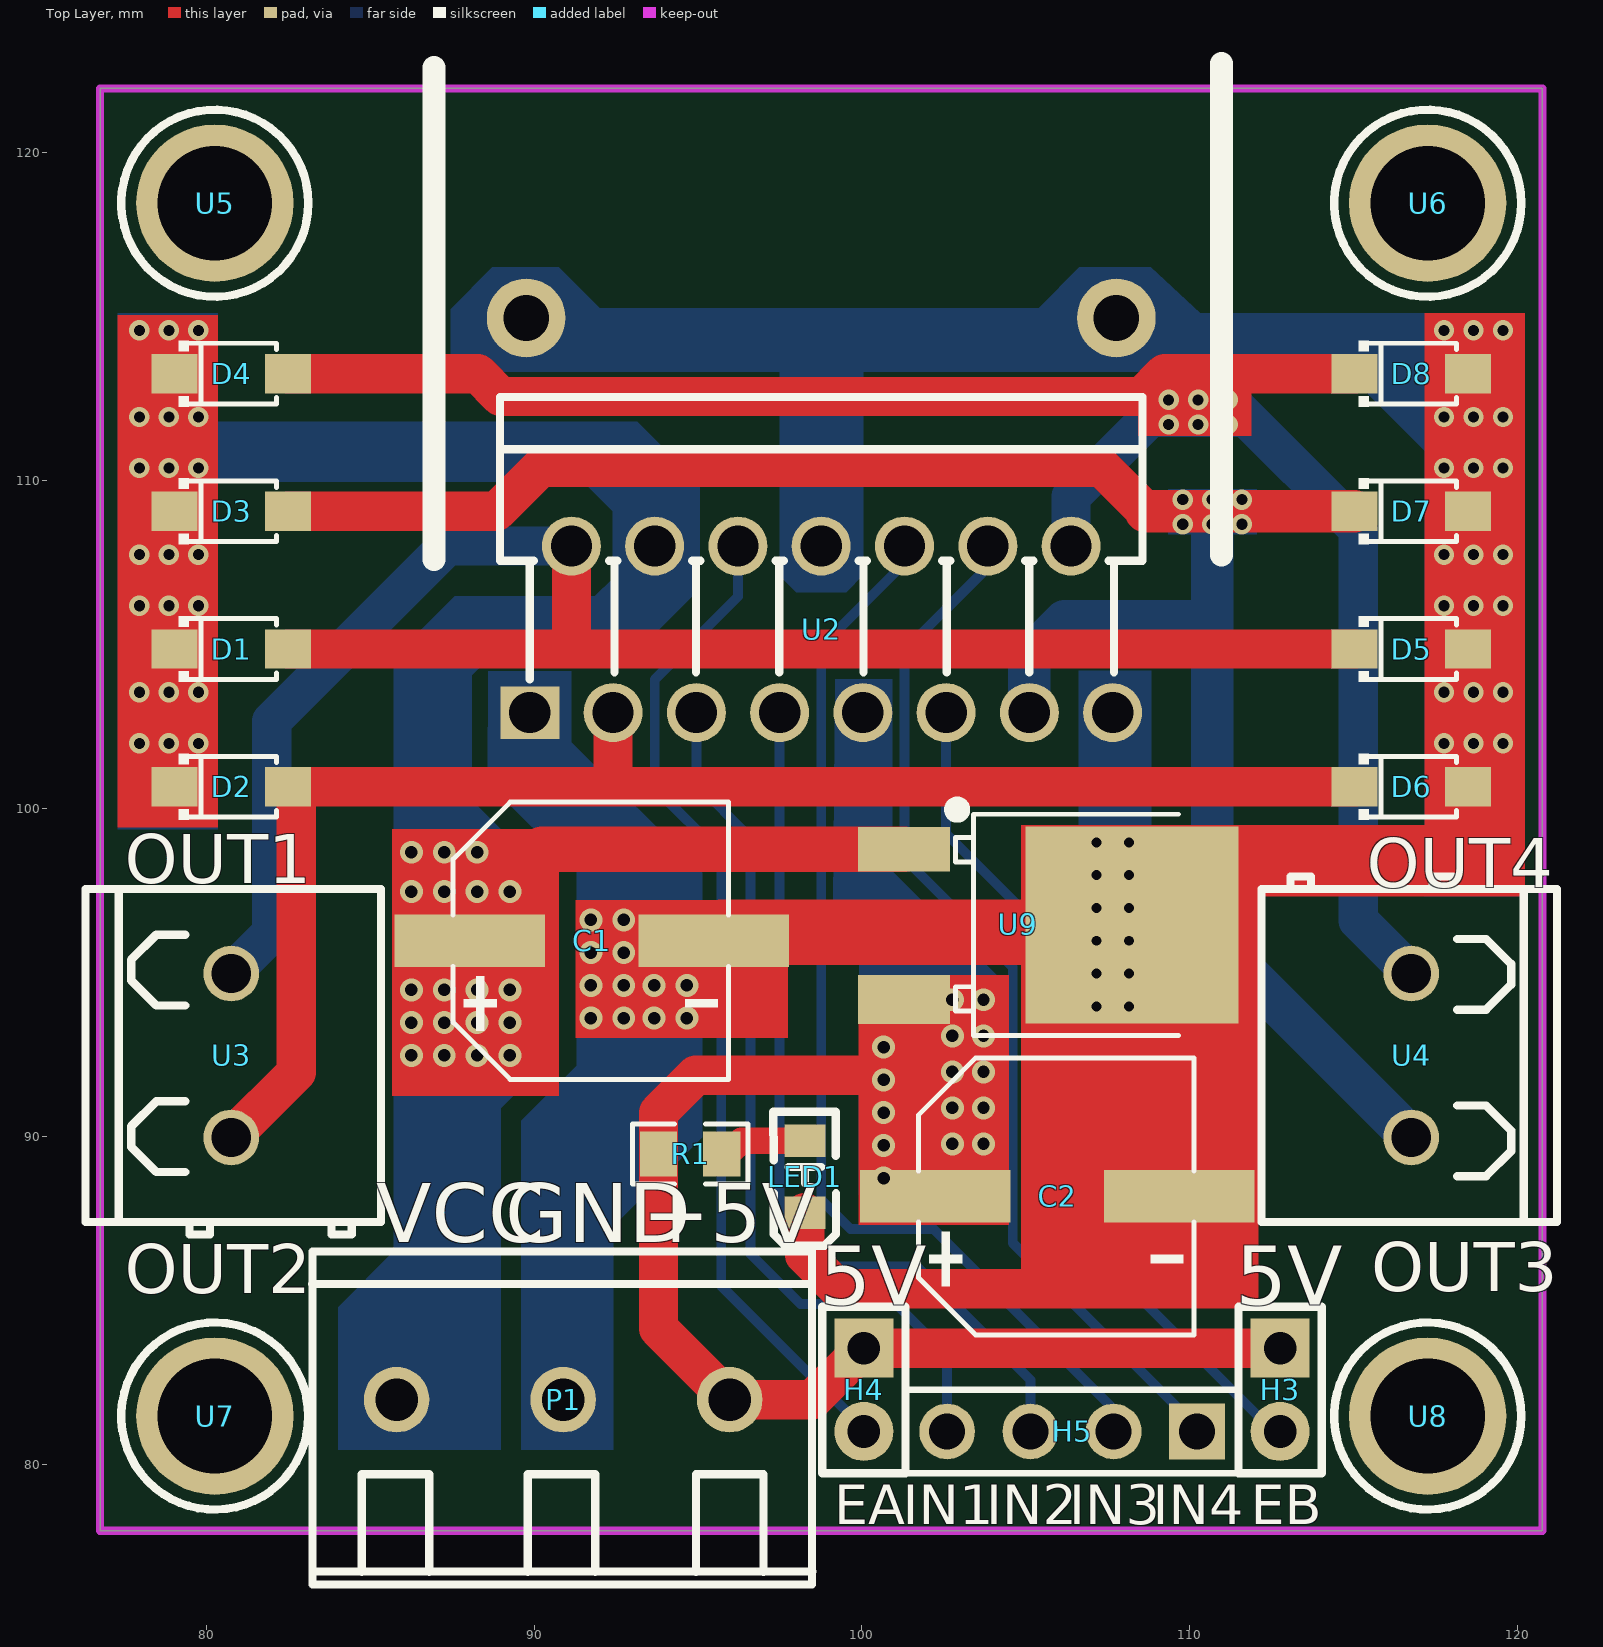
[diagram p0: Top Layer view]
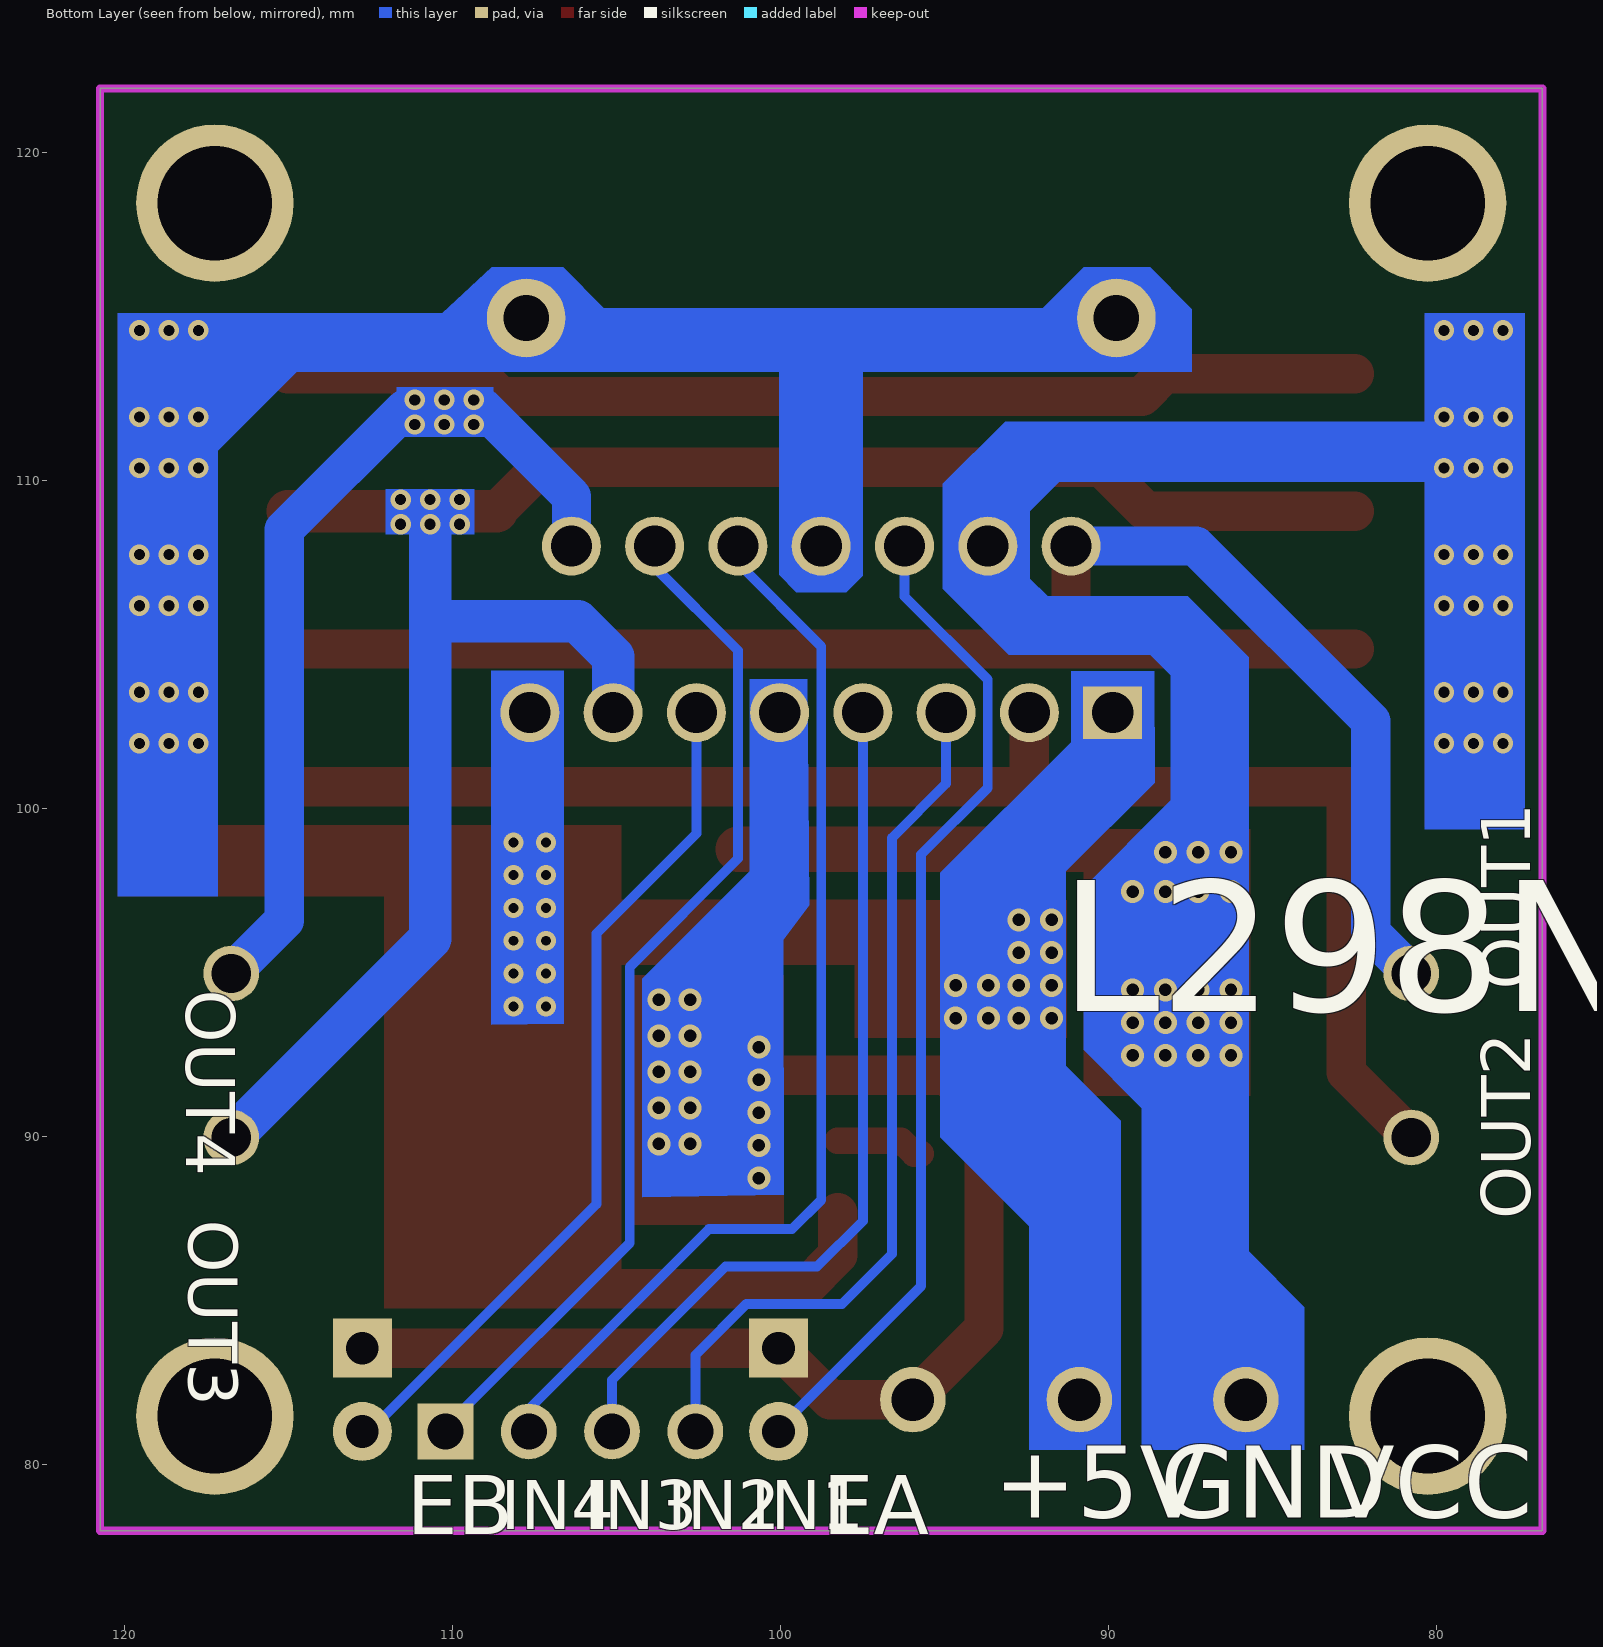
[diagram p1: Bottom Layer view, seen from below]
# Altium PCB MISC51599.pcbdoc
Units mm, origin at the board's own origin, x right, y up, seen from the top; angles counter-clockwise.
Board outline 44 x 44 mm, 2 copper layers (Top Layer, Bottom Layer), stack 1.58 mm thick; 24 components, 14 nets, 63 pads, 112 vias.

## Layer stack, top to bottom
Top Solder Mask Layer: solder mask 0.01, Dk 3.3
Top Layer: signal copper 0.035
Dielectric1: surface 1.51, FR4, Dk 4.5
Bottom Layer: signal copper 0.035
Bottom Solder Mask Layer: solder mask 0.01, Dk 3.3

## Board outline
76.76,121.966 76.76,77.966 120.76,77.966 120.76,121.966

## Design rules (kind name [scope] priority, off if disabled: settings)
BoardOutlineClearance copperThickness2oz_1 [All] p2 off: genericclearance=0.203 ignorepadtopadclearanceinfootprint=FALSE except(0: Arc-SplitContinuation Track-SplitContinuation SMDPad-SplitContinuation THPad-SplitContinuation Via-SplitContinuation Fill-SplitContinuation Region-SplitContinuation Poly-SplitContinuation Text-SplitContinuation Hole-SplitContinuation; 0.152: SMDPad-CutoutEdge THPad-CutoutEdge Via-CutoutEdge Fill-CutoutEdge Region-CutoutEdge Text-CutoutEdge Hole-CutoutEdge; 0.254: Poly-OutlineEdge Poly-CutoutEdge; 0.3: Arc-OutlineEdge Track-OutlineEdge SMDPad-OutlineEdge THPad-OutlineEdge Via-OutlineEdge Fill-OutlineEdge Region-OutlineEdge Text-OutlineEdge Hole-OutlineEdge Arc-CutoutEdge Track-CutoutEdge)
BoardOutlineClearance Plane_innerPlane_1 [All] p4 off: genericclearance=0.102 ignorepadtopadclearanceinfootprint=FALSE except(0: Arc-SplitContinuation Track-SplitContinuation SMDPad-SplitContinuation THPad-SplitContinuation Via-SplitContinuation Fill-SplitContinuation Region-SplitContinuation Poly-SplitContinuation Text-SplitContinuation Hole-SplitContinuation; 0.152: SMDPad-CutoutEdge THPad-CutoutEdge Via-CutoutEdge Fill-CutoutEdge Region-CutoutEdge Text-CutoutEdge Hole-CutoutEdge; 0.254: Poly-OutlineEdge Poly-CutoutEdge; 0.3: Arc-OutlineEdge Track-OutlineEdge SMDPad-OutlineEdge THPad-OutlineEdge Via-OutlineEdge Fill-OutlineEdge Region-OutlineEdge Text-OutlineEdge Hole-OutlineEdge Arc-CutoutEdge Track-CutoutEdge)
BoardOutlineClearance Copper_copperRegion_1 [All] p6 off: genericclearance=0.102 ignorepadtopadclearanceinfootprint=FALSE except(0: Arc-SplitContinuation Track-SplitContinuation SMDPad-SplitContinuation THPad-SplitContinuation Via-SplitContinuation Fill-SplitContinuation Region-SplitContinuation Poly-SplitContinuation Text-SplitContinuation Hole-SplitContinuation; 0.152: SMDPad-CutoutEdge THPad-CutoutEdge Via-CutoutEdge Fill-CutoutEdge Region-CutoutEdge Text-CutoutEdge Hole-CutoutEdge; 0.254: Poly-OutlineEdge Poly-CutoutEdge; 0.3: Arc-OutlineEdge Track-OutlineEdge SMDPad-OutlineEdge THPad-OutlineEdge Via-OutlineEdge Fill-OutlineEdge Region-OutlineEdge Text-OutlineEdge Hole-OutlineEdge Arc-CutoutEdge Track-CutoutEdge)
BoardOutlineClearance copperThickness1oz_1 [All] p8: genericclearance=0.102 ignorepadtopadclearanceinfootprint=FALSE except(0: Arc-SplitContinuation Track-SplitContinuation SMDPad-SplitContinuation THPad-SplitContinuation Via-SplitContinuation Fill-SplitContinuation Region-SplitContinuation Poly-SplitContinuation Text-SplitContinuation Hole-SplitContinuation; 0.152: SMDPad-CutoutEdge THPad-CutoutEdge Via-CutoutEdge Fill-CutoutEdge Region-CutoutEdge Text-CutoutEdge Hole-CutoutEdge; 0.254: Poly-OutlineEdge Poly-CutoutEdge; 0.3: Arc-OutlineEdge Track-OutlineEdge SMDPad-OutlineEdge THPad-OutlineEdge Via-OutlineEdge Fill-OutlineEdge Region-OutlineEdge Text-OutlineEdge Hole-OutlineEdge Arc-CutoutEdge Track-CutoutEdge)
Clearance copperThickness2oz [All] p1 off: gap=0.203 ignorepadtopadclearanceinfootprint=FALSE except(0.152: SMDPad-Track SMDPad-SMDPad THPad-Track SMDPad-THPad THPad-THPad Track-Via SMDPad-Via THPad-Via Via-Via Fill-Track Region-Track Fill-SMDPad Region-SMDPad Fill-THPad Region-THPad Fill-Via Region-Via Fill-Fill Fill-Region Region-Region Arc-Track Arc-SMDPad Arc-THPad Arc-Via Fill-Arc Region-Arc Arc-Arc Text-Track SMDPad-Text Text-THPad Text-Via Fill-Text Region-Text Arc-Text Text-Text Hole-Track Hole-SMDPad Hole-THPad Hole-Via Fill-Hole Region-Hole Hole-Arc Hole-Text; 0.254: Poly-Track Poly-SMDPad Poly-THPad Poly-Via Poly-Fill Poly-Region Poly-Poly Poly-Arc Poly-Text Poly-Hole)
Clearance Plane_innerPlane [All] p3 off: gap=0.102 ignorepadtopadclearanceinfootprint=FALSE except(0.152: SMDPad-Track SMDPad-SMDPad THPad-Track SMDPad-THPad THPad-THPad Track-Via SMDPad-Via THPad-Via Via-Via Fill-Track Region-Track Fill-SMDPad Region-SMDPad Fill-THPad Region-THPad Fill-Via Region-Via Fill-Fill Fill-Region Region-Region Arc-Track Arc-SMDPad Arc-THPad Arc-Via Fill-Arc Region-Arc Arc-Arc Text-Track SMDPad-Text Text-THPad Text-Via Fill-Text Region-Text Arc-Text Text-Text Hole-Track Hole-SMDPad Hole-THPad Hole-Via Fill-Hole Region-Hole Hole-Arc Hole-Text; 0.254: Poly-Track Poly-SMDPad Poly-THPad Poly-Via Poly-Fill Poly-Region Poly-Poly Poly-Arc Poly-Text Poly-Hole)
Clearance Copper_copperRegion [All] p5 off: gap=0.102 ignorepadtopadclearanceinfootprint=FALSE except(0.152: SMDPad-Track SMDPad-SMDPad THPad-Track SMDPad-THPad THPad-THPad Track-Via SMDPad-Via THPad-Via Via-Via Fill-Track Region-Track Fill-SMDPad Region-SMDPad Fill-THPad Region-THPad Fill-Via Region-Via Fill-Fill Fill-Region Region-Region Arc-Track Arc-SMDPad Arc-THPad Arc-Via Fill-Arc Region-Arc Arc-Arc Text-Track SMDPad-Text Text-THPad Text-Via Fill-Text Region-Text Arc-Text Text-Text Hole-Track Hole-SMDPad Hole-THPad Hole-Via Fill-Hole Region-Hole Hole-Arc Hole-Text; 0.254: Poly-Track Poly-SMDPad Poly-THPad Poly-Via Poly-Fill Poly-Region Poly-Poly Poly-Arc Poly-Text Poly-Hole)
Clearance copperThickness1oz [All] p7: gap=0.102 ignorepadtopadclearanceinfootprint=FALSE except(0.152: SMDPad-Track SMDPad-SMDPad THPad-Track SMDPad-THPad THPad-THPad Track-Via SMDPad-Via THPad-Via Via-Via Fill-Track Region-Track Fill-SMDPad Region-SMDPad Fill-THPad Region-THPad Fill-Via Region-Via Fill-Fill Fill-Region Region-Region Arc-Track Arc-SMDPad Arc-THPad Arc-Via Fill-Arc Region-Arc Arc-Arc Text-Track SMDPad-Text Text-THPad Text-Via Fill-Text Region-Text Arc-Text Text-Text Hole-Track Hole-SMDPad Hole-THPad Hole-Via Fill-Hole Region-Hole Hole-Arc Hole-Text; 0.254: Poly-Track Poly-SMDPad Poly-THPad Poly-Via Poly-Fill Poly-Region Poly-Poly Poly-Arc Poly-Text Poly-Hole)
DiffPairsRouting differentialPair [All] p1: maxlimit=0.152 minlimit=0.152 mostfreqgap=0.152 toplayer_minwidth=0.127 toplayer_prefwidth=0.254 toplayer_maxwidth=2.54 toplayer_mingap=0.152 toplayer_prefgap=0.152 toplayer_maxgap=0.152 bottomlayer_minwidth=0.127 bottomlayer_prefwidth=0.254 bottomlayer_maxwidth=2.54 bottomlayer_mingap=0.152 bottomlayer_prefgap=0.152 bottomlayer_maxgap=0.152 maxuncoupledlength=0.254
HoleToHoleClearance otherClearance [All] p1: gap=0.3 allowstackedmicrovias=TRUE
Length netLength [All] p1: minlimit=0 maxlimit=0
PasteMaskExpansion pasteMaskExpansion [All] p1: expansion=0
PlaneConnect innerPlane [All] p1: planeconnectstyle=Relief reliefexpansion=0.508 reliefentries=4 reliefconductorwidth=0.254 reliefairgap=0.254
PolygonConnect copperRegion [All] p1: connectstyle=Relief reliefconductorwidth=0.254 reliefentries=4 polygonreliefangle="90 Angle" airgapwidth=0.254 via.connectstyle=Relief via.reliefconductorwidth=0.254 via.reliefentries=4 via.polygonreliefangle="90 Angle" via.airgapwidth=0.254
RoutingVias viaSize [All] p1: holewidth=0.305 width=0.61 viastyle="Through Hole" minholewidth=0.3 minwidth=0.5 maxholewidth=6.3 maxwidth=10
SolderMaskExpansion solderMaskExpansion [IsVia] p1: expansion=-25.4 istentingtop=TRUE
SolderMaskExpansion solderMaskExpansion [All] p2: expansion=0.051 istentingtop=FALSE
Width copperThickness2oz_2 [All] p1 off: maxlimit=2.54 minlimit=0.203 preferedwidth=0.254
Width copperThickness1oz_2 [All] p2: maxlimit=2.54 minlimit=0.127 preferedwidth=0.254

## Components (designator, comment, footprint, x,y, rotation, side; value= is the part's Value field where it differs from the comment)
C1 "" CAP-SMD_BD8.0-L8.3-W8.3-LS9.3-FD 91.76,95.966 r0 top
C2 "" CAP-SMD_BD8.0-L8.3-W8.3-LS9.3-FD 105.96,88.166 r0 top
D1 "" SOD-123FL_L2.7-W1.8-LS3.8-RD 80.76,104.866 r0 top
D2 "" SOD-123FL_L2.7-W1.8-LS3.8-RD 80.76,100.666 r0 top
D3 "" SOD-123FL_L2.7-W1.8-LS3.8-RD 80.76,109.066 r0 top
D4 "" SOD-123FL_L2.7-W1.8-LS3.8-RD 80.76,113.266 r0 top
D5 "" SOD-123FL_L2.7-W1.8-LS3.8-RD 116.76,104.866 r0 top
D6 "" SOD-123FL_L2.7-W1.8-LS3.8-RD 116.76,100.666 r0 top
D7 "" SOD-123FL_L2.7-W1.8-LS3.8-RD 116.76,109.066 r0 top
D8 "" SOD-123FL_L2.7-W1.8-LS3.8-RD 116.76,113.266 r0 top
H3 "" HDR-TH_2P-P2.54-V-M-1 112.76,82.266 r270 top
H4 "" HDR-TH_2P-P2.54-V-M-1 100.06,82.266 r270 top
H5 "826629-4" HDR-TH_4P-P2.54-V-M-1 106.41,80.996 r180 top
LED1 "" LED0805-RD_BLUE 98.26,88.766 r90 top
P1 "" CONN-TH_3P-P5.00_WJ500V-5.08-3P 90.886,81.966 r180 top
R1 "" R0805 94.76,89.466 r180 top
U2 "L298N" multiwatt-15_l19.6-w5.0-p1.27-l 98.76,105.466 r0 top
U3 "" CONN-TH_DB302-5.0-2P 80.76,92.466 r270 top
U4 "" CONN-TH_DB302-5.0-2P 116.76,92.466 r90 top
U5 "" SMD_BD4.2-L4.7-W4.7-D3.0 80.26,118.466 r0 top
U6 "" SMD_BD4.2-L4.7-W4.7-D3.0 117.26,118.466 r0 top
U7 "" SMD_BD4.2-L4.7-W4.7-D3.0 80.26,81.466 r0 top
U8 "" SMD_BD4.2-L4.7-W4.7-D3.0 117.26,81.466 r0 top
U9 "L78M05ABDT-TR" TO-252-2_L6.5-W6.1-P4.58-LS10.0-TL 104.76,96.466 r0 top

## Footprints (in the part's own frame and the unit in brackets; to place one, negate y for a bottom-side part, rotate by r counter-clockwise, add the part's x,y. Pads: shape width x height; smd on the part's side, far side on the other; paste and mask are expansions set on the pad)
CAP-SMD_BD8.0-L8.3-W8.3-LS9.3-FD [mil]
  rect 181.1x63 smd paste+0 mask+2: 1(-146.6,0) 2(146.6,0)
  silkscreen extent -166,-166 164,166
CONN-TH_3P-P5.00_WJ500V-5.08-3P [mm]
  round 1.999 hole 1.3 paste+0 mask+0.051: 1(-5.08,0) 2(0,0) 3(5.08,0)
  silkscreen extent -7.6,-4.53 7.66,5.64
CONN-TH_DB302-5.0-2P [mm]
  round 1.7 hole 1.2 paste+0 mask+0.05: 1(-2.5,0) 2(2.5,0)
  silkscreen extent -5.08,-4.45 5.46,4.57
HDR-TH_2P-P2.54-V-M-1 [mm]
  rect 1.8x1.8 hole 1 paste+0 mask+0.051: 1(-1.27,0)
  round 1.8 hole 1 paste+0 mask+0.051: 2(1.27,0)
  silkscreen extent -2.54,-1.27 2.54,1.27
HDR-TH_4P-P2.54-V-M-1 [mm]
  rect 1.7x1.7 hole 1.1 paste+0 mask+0.051: 1(-3.81,0)
  round 1.7 hole 1.1 paste+0 mask+0.051: 2(-1.27,0) 3(1.27,0) 4(3.81,0)
  silkscreen extent -5.08,-1.27 5.08,1.27
LED0805-RD_BLUE [mm]
  rect 1.001x1.25 smd paste+0 mask+0.051: 1(-1.1,0) 2(1.1,0)
  silkscreen extent -2.1,-0.95 1.98,0.96
multiwatt-15_l19.6-w5.0-p1.27-l [mm]
  rect 1.8x1.6 hole 1.26 paste+0 mask+0.051: 1(-8.89,-2.54)
  round 1.8 hole 1.26 paste+0 mask+0.051: 2(-7.62,2.54) 3(-6.35,-2.54) 4(-5.08,2.54) 5(-3.81,-2.54) 6(-2.54,2.54) 7(-1.27,-2.54) 8(0,2.54) 9(1.27,-2.54) 10(2.54,2.54) 11(3.81,-2.54) 12(5.08,2.54) 13(6.35,-2.54) 14(7.62,2.54) 15(8.89,-2.54)
  silkscreen extent -9.8,-1.52 9.8,7.09
R0805 [mm]
  rect 1.133x1.377 smd paste-100 mask+0.051: 1(-0.966,0) 2(0.966,0)
  silkscreen extent -1.76,-0.92 1.76,0.92
SMD_BD4.2-L4.7-W4.7-D3.0 [mm]
  round 4.8 hole 3.5 paste+0 mask+0.05: 1(0,0)
  silkscreen extent -2.85,-2.85 2.85,2.85
SOD-123FL_L2.7-W1.8-LS3.8-RD [mm]
  rect 1.4x1.199 smd paste+0 mask+0.051: 1(-1.735,0) 2(1.735,0)
  silkscreen extent -1.61,-1 1.38,1
TO-252-2_L6.5-W6.1-P4.58-LS10.0-TL [mm]
  rect 2.8x1.35 smd paste+0 mask+0.051: 1(-3.475,2.29)
  rect 2.8x1.5 smd paste+0 mask+0.051: 3(-3.475,-2.29)
  rect 6.5x6 smd paste+0 mask+0.051: 4(3.475,-0.017)
  silkscreen extent -2.06,-3.39 4.9,3.7

## Free pads (board coordinates)
  round 2.4 hole 1.4 paste+0 mask+0.051: 1(89.76,114.966) 1(107.76,114.966)

## Via types
v1: diameter 0.62, hole 0.34, Top Layer to Bottom Layer, 54 vias
v2: diameter 0.7, hole 0.381, Top Layer to Bottom Layer, 46 vias
v3: diameter 0.61, hole 0.305, Top Layer to Bottom Layer, 12 vias

## Nets (pads, with @x,y where several pads share a name; then routed paths per layer and width w, separated by ;. In a path a pad name is that pad's centre, name@x,y a point inside that pad or via, vN(x,y) a via of type N, cw(c..) or ccw(c..) an arc to the next point about the centre after c; other vN are vias at no path point)
12V: C1.1 D1.1 D2.1 D3.1 D4.1 P1.3 U2.4 U9.1 | length 11
  Top Layer w1.4: 90.251,98.756 U9.1
  other v1: 77.96,101.986 78.86,101.986 79.76,101.986 77.96,103.546 78.86,103.546 79.76,103.546 77.96,106.186 78.86,106.186 79.76,106.186 77.96,107.746 78.86,107.746 79.76,107.746 77.96,110.386 78.86,110.386 79.76,110.386 77.96,111.946 78.86,111.946 79.76,111.946 77.96,114.586 78.86,114.586 79.76,114.586
  other v2: 86.26,92.466 87.26,92.466 88.26,92.466 89.26,92.466 86.26,93.466 87.26,93.466 88.26,93.466 89.26,93.466 86.26,94.466 87.26,94.466 88.26,94.466 89.26,94.466 86.26,97.466 87.26,97.466 88.26,97.466 89.26,97.466 86.26,98.666 87.26,98.666 88.26,98.666
$1N983: LED1.2 R1.1 | length 2.7
  Top Layer w0.8: R1.1 95.925,89.466 96.325,89.866 LED1.2
$1N989: D1.2 D5.1 U2.2 U3.1 | length 55.2
  Top Layer w1.2: D1.2 91.14,104.866 ; U2.2 91.14,104.866 ; D5.1 91.14,104.866
  Bottom Layer w1.2: U3.1 81.996,96.202 81.996,102.662 87.34,108.006 U2.2
$1N990: D2.2 D6.1 U2.3 U3.2 | length 46.5
  Top Layer w1.2: U3.2 82.749,91.955 82.749,100.412 D2.2 92.496,100.666 ; U2.3 92.41,100.752 92.496,100.666 ; D6.1 92.496,100.666
$1N991: D3.2 D7.1 U2.13 U4.1 | length 62.3
  Top Layer w1.2: D3.2 88.854,109.066 90.197,110.409 107.323,110.409 108.666,109.066
  Top Layer w1.3: 108.666,109.066 D7.1
  Bottom Layer w1.3: U2.13 105.11,104.627 106.193,105.71 110.486,105.71 ; v1@110.69,108.631 110.69,96.035 U4.1
  other v1: 109.79,108.673 110.69,108.673 111.59,108.673 109.79,109.423 110.69,109.423 111.59,109.423
$1N992: D4.2 D8.1 U2.14 U4.2 | length 57.9
  Top Layer w1.2: D4.2 88.283,113.266 88.981,112.568 108.539,112.568 109.237,113.266 D8.1
  Bottom Layer w1.2: U2.14 106.38,109.52 109.072,112.212 109.162,112.212 ; 111.46,112.187 115.143,108.504 115.143,96.583 U4.2
  other v1: 109.358,111.716 110.258,111.716 111.158,111.716 109.358,112.466 110.258,112.466 111.158,112.466
+5V: C2.1 H3.1 H4.1 P1.1 R1.2 U2.9 U9.3 | length 33.8
  Top Layer w1.2: 100.03,91.867 94.937,91.867 93.794,90.724 R1.2 93.794,84.138 P1.1 98.49,81.966 H4.1 H3.1
  other v2: 100.66,88.724 100.66,89.724 102.76,89.766 103.71,89.766 100.66,90.724 102.76,90.866 103.71,90.866 100.66,91.724 102.76,91.966 103.71,91.966 100.66,92.724 102.76,93.066 103.71,93.066 102.76,94.166 103.71,94.166
EA: H4.2 U2.6 | length 30.7
  Bottom Layer w0.3: U2.6 96.22,106.472 93.68,103.932 93.68,100.63 95.712,98.598 95.712,85.428 100.06,81.08 H4.2
EB: H3.2 U2.11 | length 26.3
  Bottom Layer w0.3: U2.11 102.57,99.233 105.618,96.185 105.618,87.93 112.552,80.996 H3.2
GND: C1.2 C2.2 D5.2 D6.2 D7.2 D8.2 LED1.1 P1.2 pad.1 U2.1 U2.8 U2.15 U9.4 | length 27.5
  Top Layer w1.2: LED1.1 98.26,86.38 99.291,85.348 106.866,85.348 C2.2
  Top Layer w1.4: v3(107.15,95.966) 107.752,95.966 U9.4
  Top Layer w2: C1.2 95.737,96.22 106.896,96.22 v3(107.15,95.966)
  other v1: 117.76,101.986 118.66,101.986 119.56,101.986 117.76,103.546 118.66,103.546 119.56,103.546 117.76,106.186 118.66,106.186 119.56,106.186 117.76,107.746 118.66,107.746 119.56,107.746 117.76,110.386 118.66,110.386 119.56,110.386 117.76,111.946 118.66,111.946 119.56,111.946 117.76,114.586 118.66,114.586 119.56,114.586
  other v2: 91.735,93.605 92.735,93.605 93.66,93.605 94.66,93.605 91.735,94.605 92.735,94.605 93.66,94.605 94.66,94.605 91.735,95.605 92.735,95.605 91.735,96.605 92.735,96.605
  other v3: 107.15,93.966 108.15,93.966 107.15,94.966 108.15,94.966 108.15,95.966 107.15,96.966 108.15,96.966 107.15,97.966 108.15,97.966 107.15,98.966 108.15,98.966
IN1: H5.4 U2.5 | length 26.8
  Bottom Layer w0.3: U2.5 94.95,100.757 96.601,99.106 96.601,86.406 98.125,84.882 101.046,84.882 102.6,83.328 H5.4
IN2: H5.3 U2.7 | length 26.7
  Bottom Layer w0.3: U2.7 97.49,87.422 98.887,86.025 101.681,86.025 105.14,82.566 H5.3
IN3: H5.2 U2.10 | length 33.2
  Bottom Layer w0.3: U2.10 101.3,107.488 98.76,104.948 98.76,88.057 99.649,87.168 102.189,87.168 107.68,81.677 H5.2
IN4: H5.1 U2.12 | length 31.8
  Bottom Layer w0.3: U2.12 103.84,107.361 101.3,104.821 101.3,98.471 104.602,95.169 104.602,86.749 110.22,81.131 H5.1
pads on no net: U5.1 U6.1 U7.1 U8.1

## Keep-outs
Board Outline Layer:
  the board outline again, w0.254

## Other copper
Top Layer:
  region net 12V: 77.297,115.044 77.297,99.423 80.345,99.423 80.345,115.044
  region net +5V: 99.903,94.915 99.903,87.295 104.475,87.295 104.475,94.915
  region net GND: 117.175,115.108 117.175,97.328 120.223,97.328 120.223,115.108
  region net GND: 91.267,97.201 91.267,93.01 97.744,93.01 97.744,97.201
  region net GND: 111.968,99.487 111.968,97.328 117.302,97.328 117.302,99.487
  region net 12V: 85.679,99.36 85.679,91.232 90.759,91.232 90.759,99.36
  region net GND: 104.856,99.487 104.856,84.755 112.095,84.755 112.095,99.487
  region net $1N992: 108.429,112.863 108.429,111.376 111.875,111.376 111.875,112.863
Bottom Layer:
  region net GND: 120.223,97.328 120.223,115.108 110.317,115.108 108.812,116.505 106.634,116.505 105.391,115.262 97.49,115.262 97.49,107.107 97.998,106.599 99.522,106.599 100.047,107.123 100.047,113.33 114.762,113.33 117.175,110.917 117.175,97.328
  region net GND: 101.554,115.263 92,115.263 90.759,116.505 88.727,116.505 87.457,115.235 87.457,113.33 101.554,113.33
  region net 12V: 84.028,80.437 88.981,80.437 88.981,90.863 90.759,92.641 90.759,97.582 88.092,100.249 88.092,104.059 88.727,104.694 93.045,104.694 95.048,106.697 95.048,109.901 93.143,111.806 80.345,111.806 80.345,115.108 77.297,115.108 77.297,99.36 80.345,99.36 80.345,109.965 91.498,109.965 92.398,109.066 92.398,107.016 91.854,106.472 87.584,106.472 85.724,104.612 85.724,86.487 84.028,84.791
  region net GND: 88.6,104.186 88.583,100.793 91.296,98.08 91.296,92.15 89.616,90.47 89.616,80.437 92.41,80.437 92.41,87.255 95.125,89.97 95.125,98.041 91.14,102.027 91.14,104.186
  region net +5V: 99.906,88.219 104.215,88.14 104.215,94.804 100.933,98.086 100.933,103.936 99.19,103.936 99.121,97.053 99.917,95.989
  region net GND: 106.609,93.441 108.82,93.409 108.82,104.208 106.609,104.208
  region net $1N991: 109.348,109.741 109.348,108.372 112.039,108.372 112.039,109.741
  region net $1N992: 108.764,112.855 108.764,111.344 111.705,111.344 111.705,112.855

## Silkscreen, mask and mechanical layers (free items; w line width, h text height)
Top Silkscreen Layer:
  lines w0.7: 86.943,107.601 86.943,122.601 ; 110.968,107.728 110.968,122.728
  text "OUT1" at 77.51,97.716 h1.5
  text "OUT4" at 115.406,97.598 h1.5
  text "VCC" at 85.178,86.766 h1.8
  text "GND" at 89.115,86.766 h1.8
  text "+5V" at 93.306,86.766 h1.8
  text "OUT3" at 115.533,85.279 h1.5
  text "OUT2" at 77.51,85.216 h1.5
  text "5V" at 98.71,84.866 h1.8
  text "5V" at 111.41,84.866 h1.8
  text "EA" at 99.16,78.166 h1.2
  text "IN1" at 101.25,78.166 h1.2
  text "IN2" at 103.79,78.166 h1.2
  text "IN3" at 106.33,78.166 h1.2
  text "IN4" at 108.87,78.166 h1.2
  text "EB" at 111.86,78.166 h1.2
Bottom Silkscreen Layer:
  text "OUT1" at 77.135,94.466 h1.5 r270
  text "OUT4" at 118.135,94.466 h1.5 r90
  text "L298N" at 91.487,93.808 h4
  text "OUT2" at 77.135,87.466 h1.5 r270
  text "OUT3" at 118.055,87.45 h1.5 r90
  text "VCC" at 83.331,78.366 h2.2
  text "GND" at 88.411,78.366 h2.2
  text "+5V" at 93.491,78.366 h2.2
  text "IN1" at 100.912,78.016 h1.5
  text "IN2" at 103.452,78.016 h1.5
  text "IN3" at 105.992,78.016 h1.5
  text "IN4" at 108.532,78.016 h1.5
  text "EA" at 98.71,77.866 h1.8
  text "EB" at 111.41,77.866 h1.8